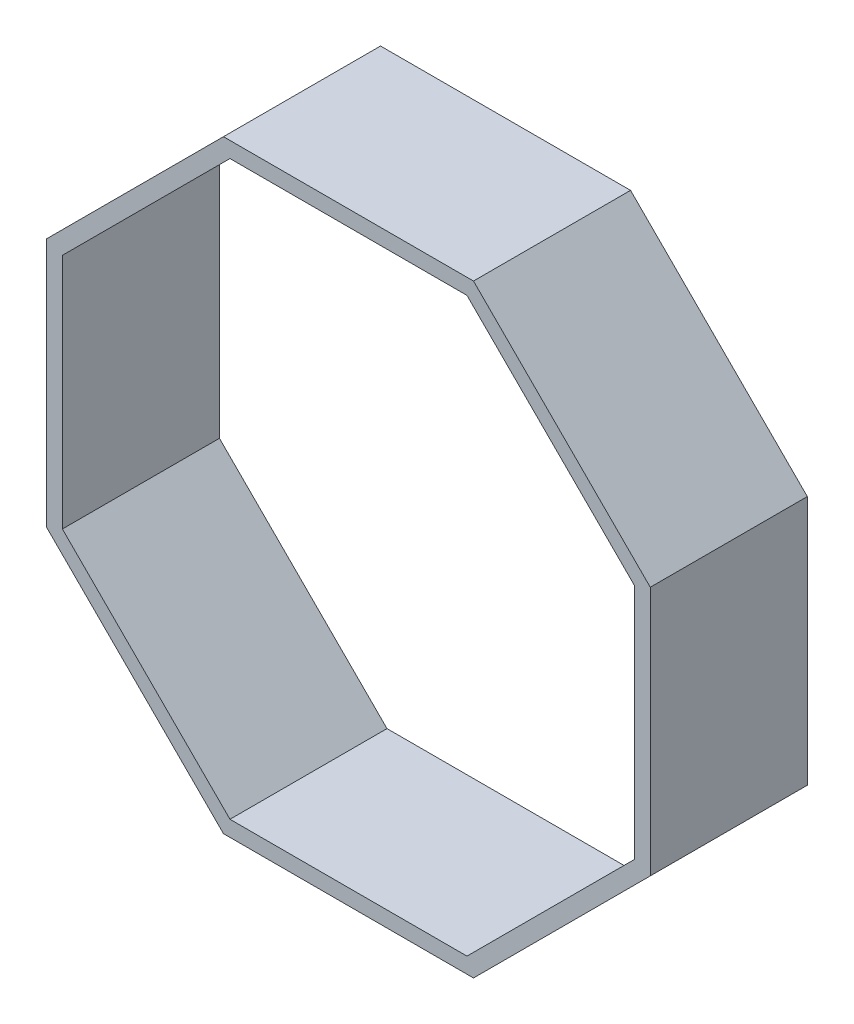
from build123d import *

# Parameters (mm, degrees)
EXTRUDE_1_DEPTH     = 50
CUT_EXTRUDE_1_DEPTH = 606


with BuildPart() as part:
    # 草图1 → 凸台-拉伸1 (new body)
    with BuildSketch(Plane.XY):
        Polygon((-39.799076966, 96.083471381), (-96.083471381, 39.799076966), (-96.083471381, -39.799076966), (-39.799076966, -96.083471381), (39.799076966, -96.083471381), (96.083471381, -39.799076966), (96.083471381, 39.799076966), (39.799076966, 96.083471381), align=None)
    extrude(amount=EXTRUDE_1_DEPTH)

    # 草图2 → 切除-拉伸1 (cut)
    with BuildSketch(Plane.XY.offset(50)):
        Polygon((37.728009154, 91.083471381), (-37.728009154, 91.083471381), (-91.083471381, 37.728009154), (-91.083471381, -37.728009154), (-37.728009154, -91.083471381), (37.728009154, -91.083471381), (91.083471381, -37.728009154), (91.083471381, 37.728009154), align=None)
    extrude(amount=-CUT_EXTRUDE_1_DEPTH, mode=Mode.SUBTRACT)


solid = part.part
